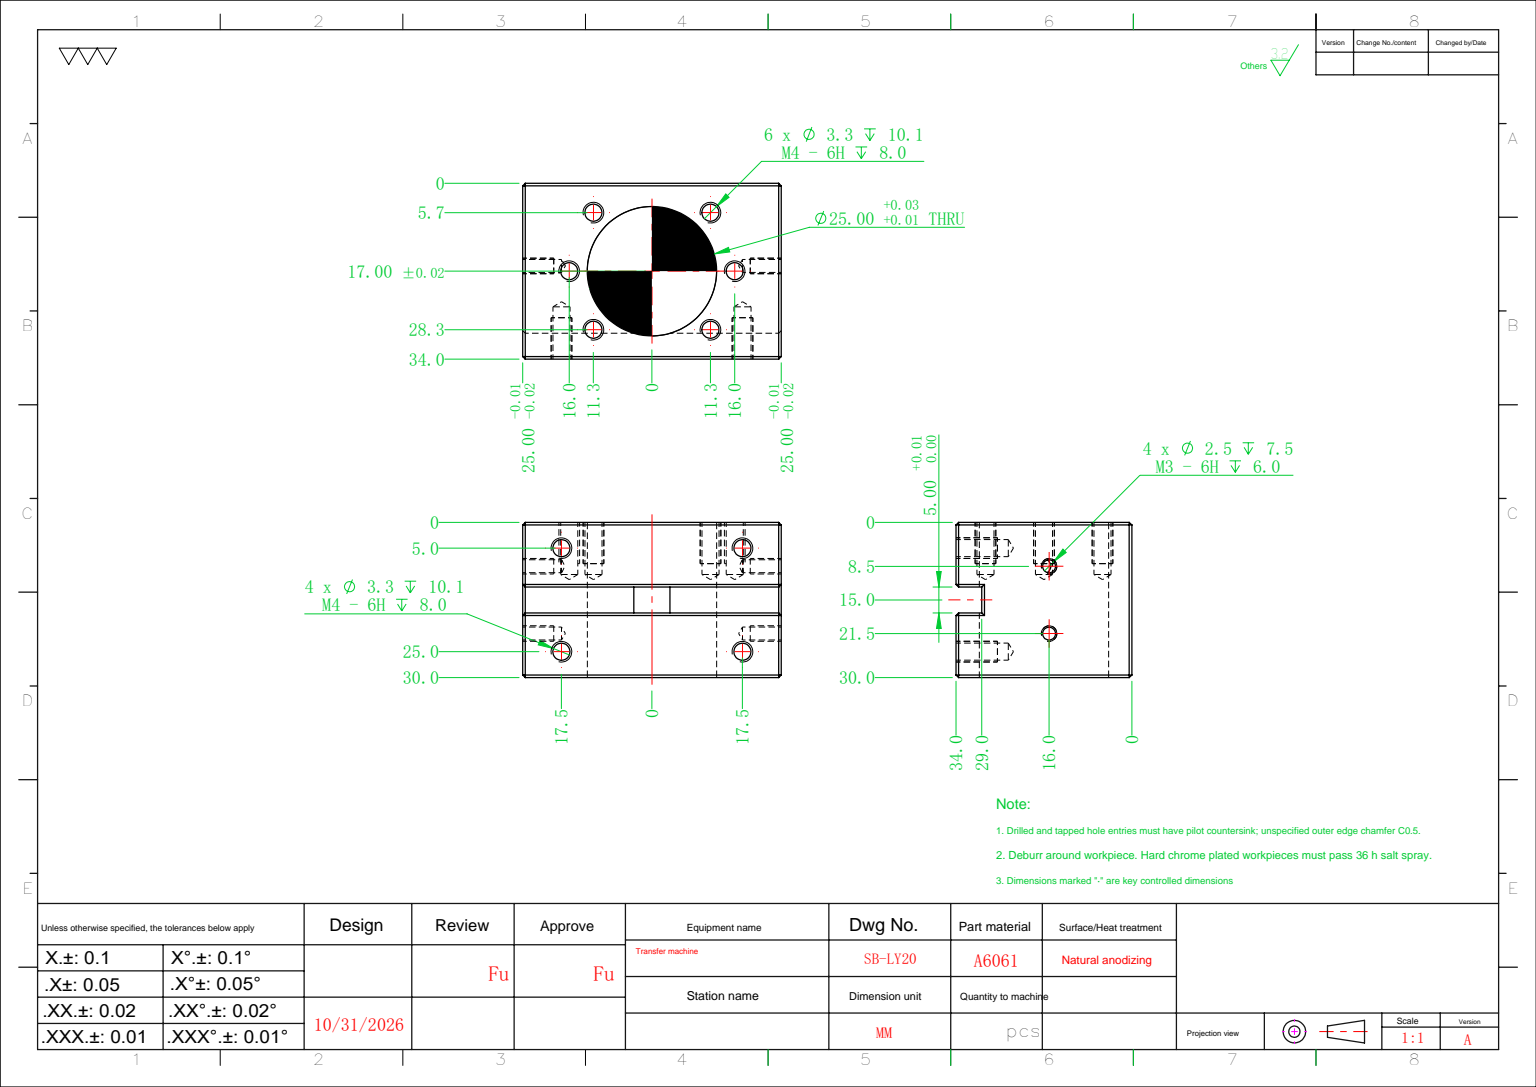
from build123d import *

# Parameters (mm, degrees)
SKETCH_1_W                  = 50
SKETCH_1_H                  = 34
EXTRUDE_1_DEPTH             = 30
HOLE_WIZARD_M4_1_D          = 3.3
HOLE_WIZARD_M4_1_DEPTH      = 10.1
HOLE_WIZARD_M4_1_TIP        = 0.991420021
HOLE_WIZARD_M3_1_AT_2_COUNT = 2
HOLE_WIZARD_M3_1_AT_2_PITCH = 13
SKETCH_15_R                 = 12.5
CUT_EXTRUDE_1_DEPTH         = 43.591079007
HOLE_WIZARD_M4_2_D          = 3.3
HOLE_WIZARD_M4_2_DEPTH      = 10.1
HOLE_WIZARD_M4_2_TIP        = 0.991420021
SKETCH_18_W                 = 50
SKETCH_18_H                 = 5
CUT_EXTRUDE_2_DEPTH         = 5
CHAMFER_1_SIZE              = 0.5


with BuildPart() as part:
    # 草图1 → 凸台-拉伸1 (new body)
    with BuildSketch(Plane.XY):
        Rectangle(SKETCH_1_W, SKETCH_1_H)
    extrude(amount=EXTRUDE_1_DEPTH)

    # M4 螺纹孔1
    with Locations(Plane(origin=(0, 0, 0), x_dir=(-1, 0, 0), z_dir=(0, 0, -1))):
        with Locations((-11.313708499, -11.313708499), (-16, 0), (-11.313708499, 11.313708499), (11.313708499, 11.313708499), (16, 0), (11.313708499, -11.313708499)):
            Hole(HOLE_WIZARD_M4_1_D / 2, depth=HOLE_WIZARD_M4_1_DEPTH)
            with Locations((0, 0, -(HOLE_WIZARD_M4_1_DEPTH + HOLE_WIZARD_M4_1_TIP / 2))):  # 118° drill point
                Cone(0, HOLE_WIZARD_M4_1_D / 2, HOLE_WIZARD_M4_1_TIP, mode=Mode.SUBTRACT)

    # 草图12 → M3 螺纹孔1 (revolve, cut)
    with BuildSketch(Plane(origin=(-25, -1, 8.5), x_dir=(0, 0, 1), z_dir=(0, 1, 0))):
        Polygon((0, 0), (0, 8.251075774), (1.25, 7.5), (1.25, 0), align=None)
    hole_wizard_m3_1 = revolve(axis=Axis((-31.35, -1, 8.5), (1, 0, 0)), mode=Mode.SUBTRACT)

    # M3 螺纹孔1 at 2: M3 螺纹孔1 ×2
    with Locations(*[(0, 0, i * HOLE_WIZARD_M3_1_AT_2_PITCH) for i in range(1, HOLE_WIZARD_M3_1_AT_2_COUNT)]):
        add(hole_wizard_m3_1, mode=Mode.SUBTRACT)

    # 镜向1: M3 螺纹孔1 across plane
    add(hole_wizard_m3_1.mirror(Plane(origin=(0, 0, 0), x_dir=(0, 0, 1), z_dir=(1, 0, 0))), mode=Mode.SUBTRACT)

    # 镜向1 copy 1 sketch → 镜向1 copy 1 (revolve, cut)
    with BuildSketch(Plane(origin=(25, -1, 21.5), x_dir=(0, 0, 1), z_dir=(0, 1, 0))):
        Polygon((0, 0), (0, -8.251075774), (1.25, -7.5), (1.25, 0), align=None)
    revolve(axis=Axis((31.35, -1, 21.5), (1, 0, 0)), mode=Mode.SUBTRACT)

    # 草图15 → 切除-拉伸1 (cut, through all)
    with BuildSketch(Plane.XY.offset(30)):
        Circle(SKETCH_15_R)
    extrude(amount=-CUT_EXTRUDE_1_DEPTH, mode=Mode.SUBTRACT)

    # M4 螺纹孔2
    with Locations(Plane(origin=(0, 17, 0), x_dir=(1, 0, 0), z_dir=(0, 1, 0))):
        with Locations((17.5, -25), (-17.5, -25), (-17.5, -5), (17.5, -5)):
            Hole(HOLE_WIZARD_M4_2_D / 2, depth=HOLE_WIZARD_M4_2_DEPTH)
            with Locations((0, 0, -(HOLE_WIZARD_M4_2_DEPTH + HOLE_WIZARD_M4_2_TIP / 2))):  # 118° drill point
                Cone(0, HOLE_WIZARD_M4_2_D / 2, HOLE_WIZARD_M4_2_TIP, mode=Mode.SUBTRACT)

    # 草图18 → 切除-拉伸2 (cut)
    with BuildSketch(Plane(origin=(0, 17, 0), x_dir=(1, 0, 0), z_dir=(0, 1, 0))):
        with Locations((0, -15)):
            Rectangle(SKETCH_18_W, SKETCH_18_H)
    extrude(amount=-CUT_EXTRUDE_2_DEPTH, mode=Mode.SUBTRACT)

    # 倒角1
    chamfer_1_edges = [part.edges().sort_by_distance(p)[0] for p in [
        (-25, 0, 30),
        (0, 17, 17.5),
        (0, -17, 30),
        (25, 0, 30),
        (0, -17, 0),
        (-25, 0, 0),
        (0, 17, 0),
        (25, 0, 0),
        (0, 17, 30),
        (25, -17, 15),
        (-25, -17, 15),
        (-25, 17, 23.75),
        (25, 17, 23.75),
        (-25, 17, 6.25),
        (25, 17, 6.25),
        (25, 14.5, 17.5),
        (-25, 14.5, 12.5),
        (25, 12, 15),
        (25, 14.5, 12.5),
        (-25, 12, 15),
        (-25, 14.5, 17.5),
        (0, 17, 12.5),
    ]]
    chamfer(chamfer_1_edges, length=CHAMFER_1_SIZE)


solid = part.part
